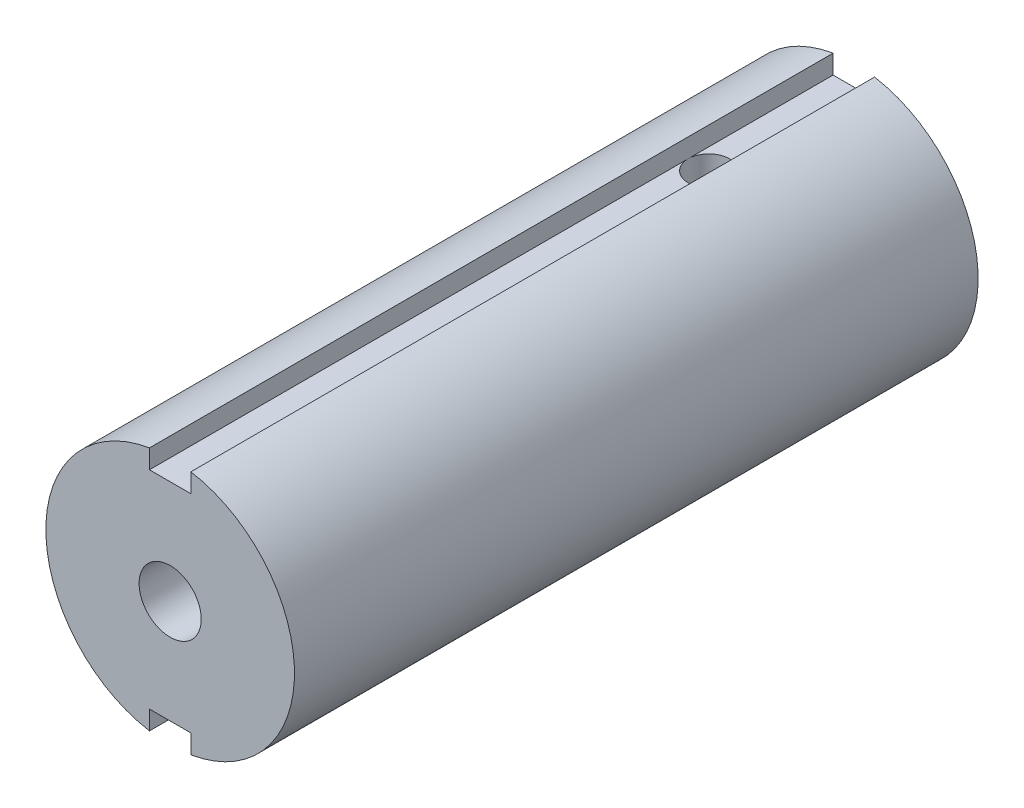
SolidWorks part; units mm, degrees
material "AISI 类型 316L 不锈钢"
ref_plane "Front Plane" through (0, 0, 0) normal (0, 0, 1) x (1, 0, 0)
ref_plane "Top Plane" through (0, 0, 0) normal (0, 1, 0) x (1, 0, 0)
ref_plane "Right Plane" through (0, 0, 0) normal (1, 0, 0) x (0, 0, -1)
sketch "Sketch1" plane through (0, 0, 0) normal (0, 0, 1) x (1, 0, 0)
  circle A0 centre (0, 0) radius 6
extrude "Boss-Extrude1" add sketch "Sketch1" along normal blind 33
sketch "Sketch2" plane through (0, 0, 33) normal (0, 0, 1) x (1, 0, 0)
  line L1 (1, 7) -> (-1, 7)
  line L2 (1, 7) -> (1, 5)
  line L3 (1, 5) -> (-1, 5)
  line L4 (-1, 7) -> (-1, 5)
  line L5 (1, 7) -> (-1, 5) construction
  line L6 (1, 5) -> (-1, 7) construction
  circle A0 centre (0, 0) radius 6 construction
  point P0 (0, 6)
extrude "Cut-Extrude1" cut sketch "Sketch2" against normal blind 33
mirror "Mirror1" about plane through (0, 0, 0) normal (0, 1, 0) of "Cut-Extrude1"
sketch "Sketch3" plane through (0, 0, 33) normal (0, 0, 1) x (1, 0, 0)
  circle A0 centre (0, 0) radius 1.5
extrude "Cut-Extrude2" cut sketch "Sketch3" against normal blind 23
sketch "Sketch4" plane through (0, 5, 0) normal (0, 1, 0) x (1, 0, 0)
  line L0 (0, 0) -> (0, -7) construction
  line L1 (-1, 0) -> (1, 0) construction
  circle A0 centre (0, -7) radius 1
extrude "Cut-Extrude3" cut sketch "Sketch4" against normal blind 7
sketch "Sketch5" plane through (0, 0, 0) normal (0, 0, -1) x (-1, 0, 0)
  circle A0 centre (0, 0) radius 3.5
extrude "Cut-Extrude4" cut sketch "Sketch5" against normal blind 2
sketch "Sketch6" plane through (0, 0, 2) normal (0, 0, -1) x (-1, 0, 0)
  circle A0 centre (0, 0) radius 3.4
extrude "Boss-Extrude2" add sketch "Sketch6" along normal blind 2
